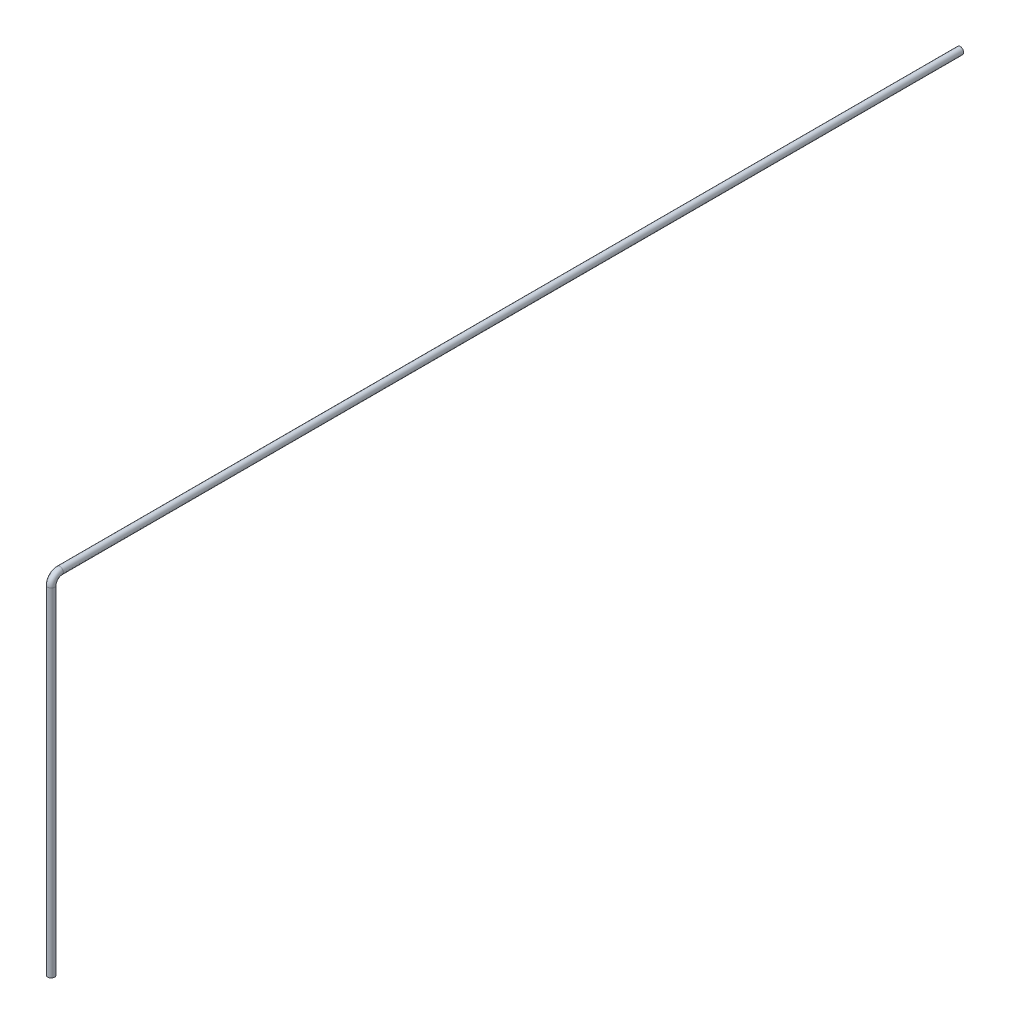
from build123d import *

# Parameters (mm, degrees)
SKETCH1_R   = 4
SKETCH1_R_2 = 3


with BuildPart() as part:
    # Sweep1: sweep along a path in Sketch2
    with BuildLine(Plane(origin=(0, 0, 0), x_dir=(0, 0, -1), z_dir=(1, 0, 0))) as sweep1_path:
        Line((0, 0), (0, 390))
        ThreePointArc((0, 390), (2.928932188, 397.071067812), (10, 400))
        Line((10, 400), (1050, 400))
    # Sketch1 → Sweep1 (sweep)
    with BuildSketch(Plane(origin=(0, 0, 0), x_dir=(1, 0, 0), z_dir=(0, 1, 0))):
        Circle(SKETCH1_R)
        Circle(SKETCH1_R_2, mode=Mode.SUBTRACT)
    sweep(path=sweep1_path.line)


solid = part.part
